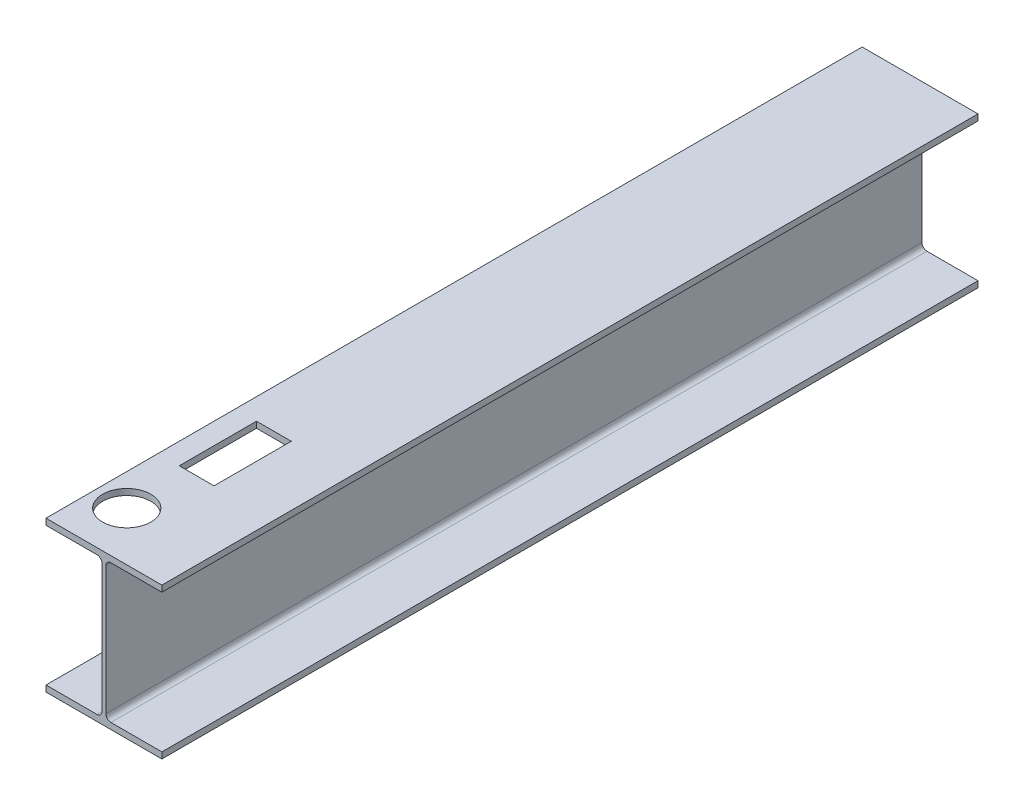
SolidWorks part; units mm, degrees
material "Q235"
ref_plane "Front Plane" through (0, 0, 0) normal (0, 0, 1) x (1, 0, 0)
ref_plane "Top Plane" through (0, 0, 0) normal (0, 1, 0) x (1, 0, 0)
ref_plane "Right Plane" through (0, 0, 0) normal (1, 0, 0) x (0, 0, -1)
sketch "Sketch1" plane through (0, 0, 0) normal (0, 0, 1) x (1, 0, 0)
  line L0 (0, 0) -> (300, 0)
  line L1 (300, 0) -> (300, 16)
  line L2 (300, 16) -> (168, 16)
  line L3 (155, 29) -> (155, 361)
  line L4 (168, 374) -> (300, 374)
  line L5 (300, 374) -> (300, 390)
  line L6 (300, 390) -> (0, 390)
  line L7 (0, 390) -> (0, 374)
  line L8 (0, 374) -> (132, 374)
  line L9 (145, 361) -> (145, 29)
  line L10 (132, 16) -> (0, 16)
  line L11 (0, 16) -> (0, 0)
  line L12 (150, 390) -> (150, 0) construction
  arc A0 (168, 16) -> (155, 29) centre (168, 29) cw
  arc A1 (145, 29) -> (132, 16) centre (132, 29) cw
  arc A2 (155, 361) -> (168, 374) centre (168, 361) cw
  arc A3 (132, 374) -> (145, 361) centre (132, 361) cw
  point P21 (155, 374)
  dimension "D7" = 13
  dimension "D1" = 390
  dimension "D2" = 300
  dimension "D3" = 10
  dimension "D4" = 5
  dimension "D5" = 16
  dimension "D6" = 16
extrude "Boss-Extrude1" add sketch "Sketch1" along normal blind 2113
sketch "Sketch2" plane through (0, 390, 0) normal (0, 1, 0) x (1, 0, 0)
  line L0 (300, -2113) -> (0, -2113) construction
  line L1 (145, -1623) -> (55, -1623)
  line L2 (145, -1623) -> (145, -1823)
  line L3 (145, -1823) -> (55, -1823)
  line L4 (55, -1623) -> (55, -1823)
  line L5 (0, -2113) -> (0, 0) construction
  line L6 (145, -2113) -> (145, 0) construction
  circle A0 centre (82, -1986) radius 62.5
  dimension "D1" = 127
  dimension "D2" = 125
  dimension "D3" = 82
  dimension "D4" = 200
  dimension "D5" = 90
  dimension "D6" = 0
  dimension "D7" = 163
extrude "Cut-Extrude1" cut sketch "Sketch2" against normal up to next
sketch "Sketch3" plane through (145, 0, 0) normal (-1, 0, 0) x (0, 0, 1)
  line L0 (2113, 361) -> (2113, 29) construction
  line L1 (1823, 390) -> (1623, 390) construction
  circle A0 centre (1723, 315) radius 25.5
  dimension "D1" = 390
  dimension "D2" = 75
  dimension "D3" = 51
extrude "Cut-Extrude2" cut sketch "Sketch3" against normal up to next
